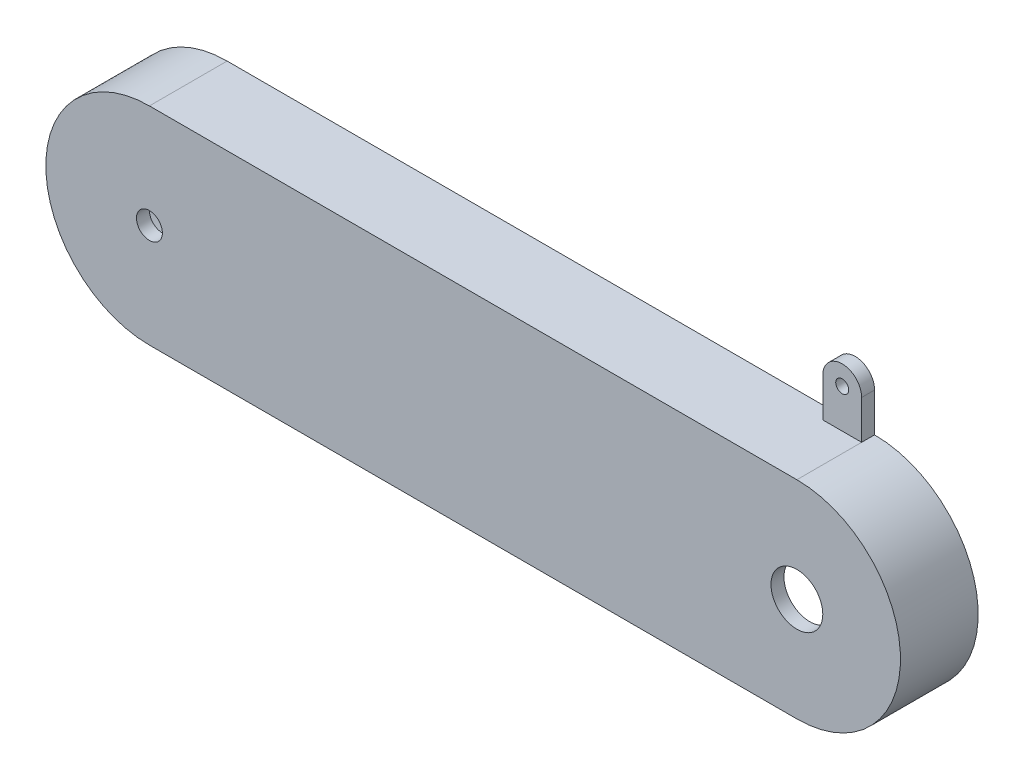
from build123d import *

# Parameters (mm, degrees)
SKETCH_1_R      = 20
SKETCH_1_R_2    = 10
EXTRUDE_1_DEPTH = 10
EXTRUDE_START   = 50
EXTRUDE_2_DEPTH = 50
SKETCH_4_R      = 5
EXTRUDE_3_DEPTH = 10


with BuildPart() as part:
    # 草图1 → 凸台-拉伸1 (new body)
    with BuildSketch(Plane.XY):
        with BuildLine():
            Line((0, 80), (-500, 80))
            ThreePointArc((-500, 80), (-580, 0), (-500, -80))
            Line((-500, -80), (0, -80))
            ThreePointArc((0, -80), (80, 0), (0, 80))
        make_face()
        Circle(SKETCH_1_R, mode=Mode.SUBTRACT)
        with Locations((-500, 0)):
            Circle(SKETCH_1_R_2, mode=Mode.SUBTRACT)
    extrude(amount=EXTRUDE_1_DEPTH)

    # 草图2 → 凸台-拉伸2 (add)
    with BuildSketch(Plane(origin=(0, 0, 0), x_dir=(-1, 0, 0), z_dir=(0, 0, -1)).offset(EXTRUDE_START)):
        with BuildLine():
            Line((0, -80), (500, -80))
            ThreePointArc((500, -80), (580, 0), (500, 80))
            Line((500, 80), (0, 80))
            ThreePointArc((0, 80), (-80, 0), (0, -80))
        make_face()
        with BuildLine():
            Line((0, -70), (500, -70))
            ThreePointArc((500, -70), (570, 0), (500, 70))
            Line((500, 70), (0, 70))
            ThreePointArc((0, 70), (-70, 0), (0, -70))
        make_face(mode=Mode.SUBTRACT)
    extrude(amount=-EXTRUDE_2_DEPTH)

    # 草图4 → 凸台-拉伸3 (add)
    with BuildSketch(Plane(origin=(0, 0, -50), x_dir=(-1, 0, 0), z_dir=(0, 0, -1))):
        with BuildLine():
            Line((0, 110), (0, 80))
            Line((0, 80), (30, 80))
            Line((30, 80), (30, 110))
            ThreePointArc((30, 110), (15, 125), (0, 110))
        make_face()
        with Locations((15, 110)):
            Circle(SKETCH_4_R, mode=Mode.SUBTRACT)
    extrude(amount=-EXTRUDE_3_DEPTH)


solid = part.part
